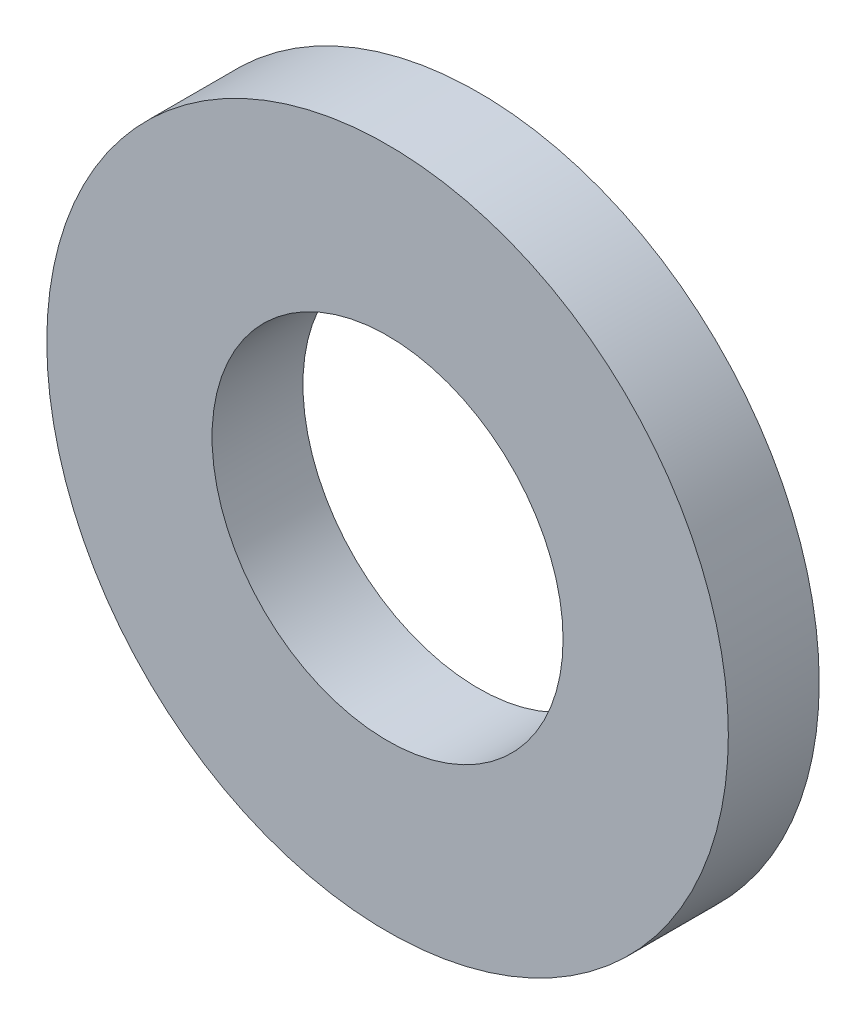
from build123d import *

# Parameters (mm, degrees)
SKETCH1_R          = 6
SKETCH1_R_2        = 3.09
BASE_EXTRUDE_DEPTH = 1.6


with BuildPart() as part:
    # Sketch1 → Base-Extrude (new body)
    with BuildSketch(Plane.XY):
        Circle(SKETCH1_R)
        Circle(SKETCH1_R_2, mode=Mode.SUBTRACT)
    extrude(amount=-BASE_EXTRUDE_DEPTH)


solid = part.part
